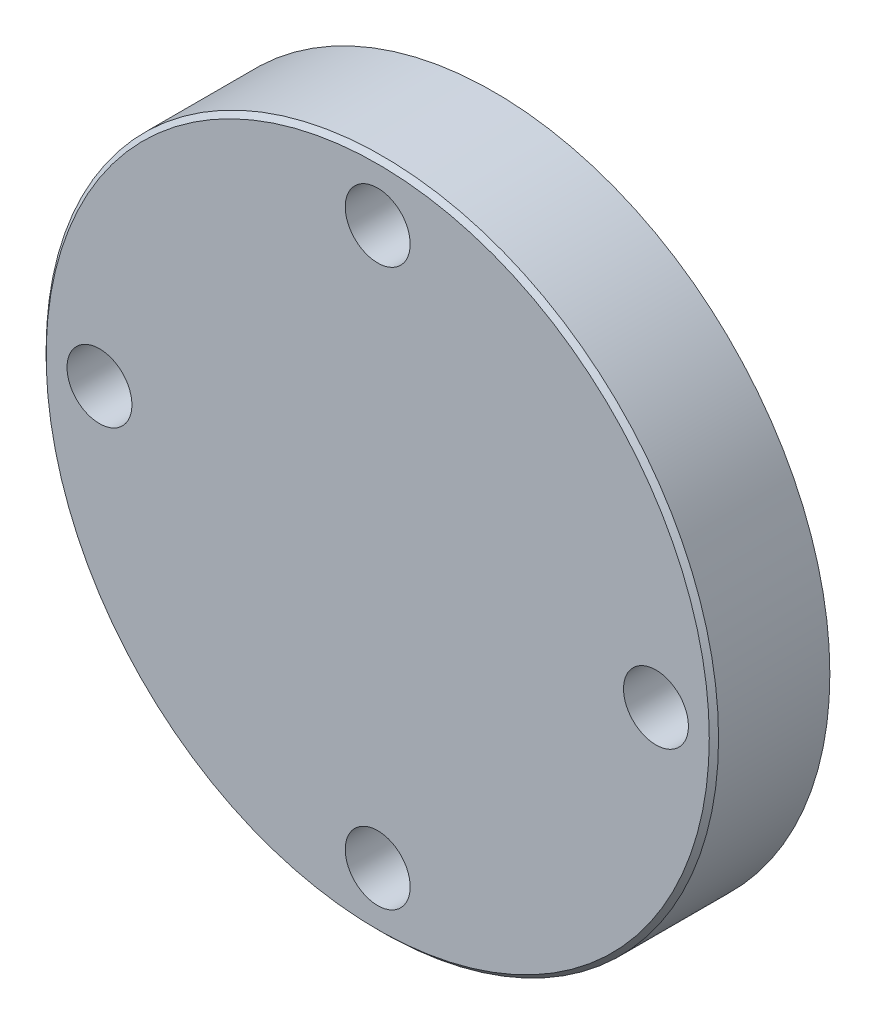
SolidWorks part; units mm, degrees
material "Q345"
ref_plane "前视基准面" through (0, 0, 0) normal (0, 0, 1) x (1, 0, 0)
ref_plane "上视基准面" through (0, 0, 0) normal (0, 1, 0) x (1, 0, 0)
ref_plane "右视基准面" through (0, 0, 0) normal (1, 0, 0) x (0, 0, -1)
sketch "草图1" plane through (0, 0, 0) normal (0, 0, 1) x (1, 0, 0)
  circle A0 centre (0, 0) radius 72.5
  dimension "D1" = 145
extrude "凸台-拉伸1" add sketch "草图1" along normal blind 25
sketch "草图2" plane through (0, 0, 25) normal (0, 0, 1) x (1, 0, 0)
  circle A0 centre (0, 0) radius 60 construction
  circle A1 centre (0, 60) radius 7
  circle A2 centre (60, 0) radius 7
  circle A3 centre (0, -60) radius 7
  circle A4 centre (-60, 0) radius 7
  point P14 (0, 0)
  dimension "D1" = 120
  dimension "D2" = 14
  dimension "D3" = 4
extrude "切除-拉伸1" cut sketch "草图2" against normal through all
sketch "草图3" plane through (0, 0, 0) normal (0, 0, -1) x (-1, 0, 0)
  line L0 (-32.5, 36) -> (32.5, 36)
  line L1 (0, 0) -> (0, 48.5) construction
  line L2 (-48.5, 0) -> (48.5, 0) construction
  line L3 (-32.5, -36) -> (32.5, -36)
  arc A0 (-32.5, 36) -> (-32.5, -36) centre (0, 0) ccw
  arc A1 (32.5, -36) -> (32.5, 36) centre (0, 0) ccw
  dimension "D1" = 97
  dimension "D2" = 72
extrude "切除-拉伸2" cut sketch "草图3" against normal blind 15
chamfer "倒角1" distance 1 angle 45 1 edges at (72.5, 0, 25)
chamfer "倒角2" distance 1 angle 45 4 edges at (0, 36, 0) (-48.5, 0, 0) (0, -36, 0) (48.5, 0, 0)
